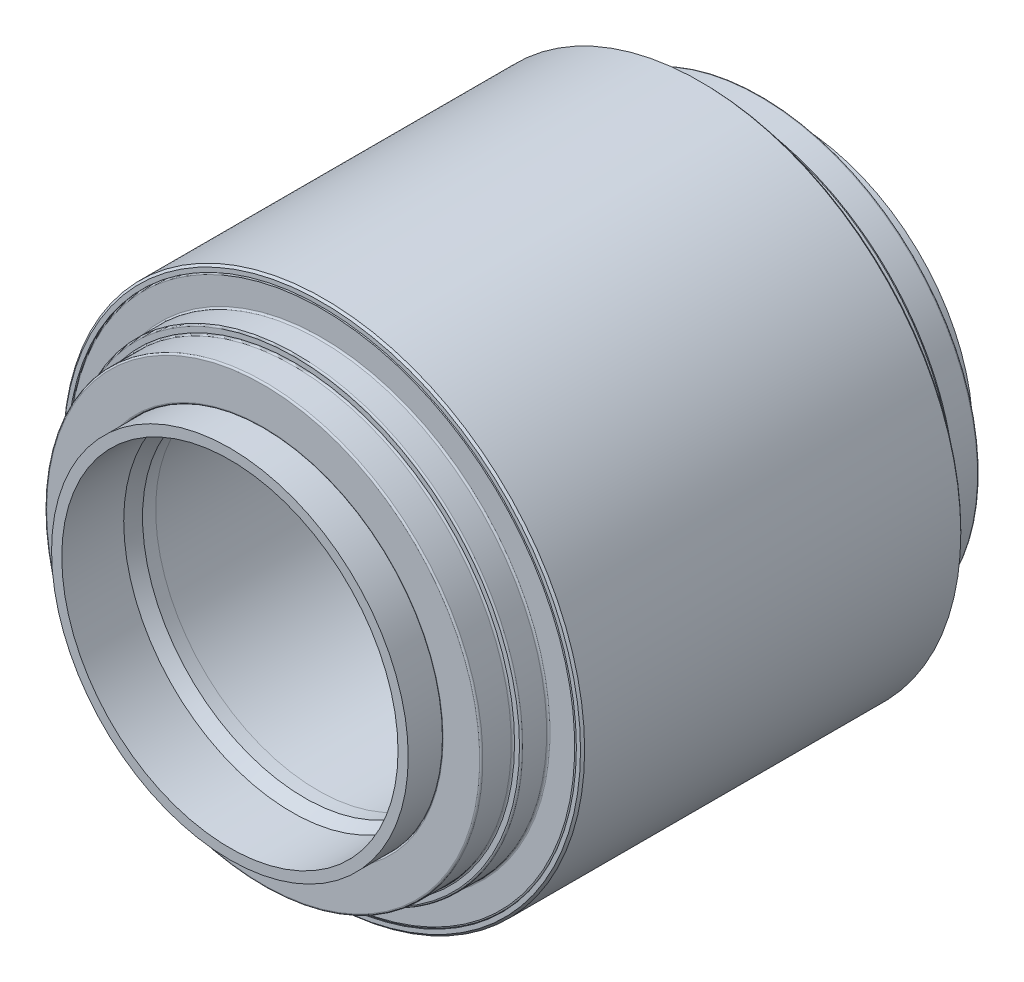
from build123d import *

# Parameters (mm, degrees)
SKETCH2_W          = 30
SKETCH2_H          = 5
SKETCH5_W          = 15.31
SKETCH5_H          = 17.764999952
SKETCH11_W         = 15.013
SKETCH11_H         = 17.764999952
FILLET1_R          = 0.8
FILLET2_R          = 0.8
CHAMFER1_SIZE      = 1
CIRPATTERN5_COUNT  = 26
CIRPATTERN7_COUNT  = 26
SKETCH15_R         = 3
CUT_EXTRUDE3_DEPTH = 225.788354196


with BuildPart() as part:
    # Sketch2 → Revolve1 (revolve)
    with BuildSketch(Plane(origin=(0, 0, 0), x_dir=(0, 0, -1), z_dir=(1, 0, 0)), mode=Mode.PRIVATE) as revolve1_sk:
        with Locations((0, 81.0749)):
            Rectangle(SKETCH2_W, SKETCH2_H)
    revolve(revolve1_sk.sketch.rotate(Axis((0, 0, 191.063546837), (0, 0, -1)), 90), axis=Axis((0, 0, 191.063546837), (0, 0, -1)))


with BuildPart() as body_2:
    # Sketch3 → Revolve2 (revolve)
    with BuildSketch(Plane(origin=(0, 0, 0), x_dir=(0, 0, -1), z_dir=(1, 0, 0)), mode=Mode.PRIVATE) as revolve2_sk:
        Polygon((-22.009341225, 88.613727462), (-71.184928734, 97.669414462), (-71.980821721, 93.5749), (-94.032, 93.5749), (-94.032, 78.5749), (-15, 78.5749), (-15, 86.5749), (-22.405649137, 86.5749), align=None)
    revolve(revolve2_sk.sketch.rotate(Axis((0, 0, 191.063546837), (0, 0, -1)), 90), axis=Axis((0, 0, 191.063546837), (0, 0, -1)))

    # Sketch7 → Revolve7 (revolve)
    with BuildSketch(Plane(origin=(0, 0, 0), x_dir=(0, 0, -1), z_dir=(-0.9927090359250009, 0.12053534748303266, 0)), mode=Mode.PRIVATE) as revolve7_sk:
        Polygon((-71.184928734, -96.95731027), (-22.009341225, -87.967647959), (-20.004670612, -98.205591502), (-69.086029785, -107.676482194), align=None)
    revolve7 = revolve(revolve7_sk.sketch.rotate(Axis((12.978822197, 106.891416831, 69.086029785), (-0.022837582945864243, -0.18808652749964044, -0.9818869094647906)), 353.201212474), axis=Axis((12.978822197, 106.891416831, 69.086029785), (-0.022837582945864243, -0.18808652749964044, -0.9818869094647906)))

    # CirPattern5: Revolve7 ×26 about axis
    cirpattern5_axis = Axis((0, 0, 191.063546837), (0, 0, -1))
    for i in range(1, CIRPATTERN5_COUNT):
        add(revolve7.rotate(cirpattern5_axis, i * 360 / CIRPATTERN5_COUNT))


with BuildPart() as body_3:
    # Sketch4 → Revolve3 (revolve)
    with BuildSketch(Plane(origin=(0, 0, 0), x_dir=(0, 0, -1), z_dir=(1, 0, 0)), mode=Mode.PRIVATE) as revolve3_sk:
        Polygon((-94.032, 78.5749), (-94.032, 85.485113365), (-104.032, 86.36), (-136.652, 86.36), (-136.652, 81.419999974), (-106.652, 81.419999974), (-100.382, 78.5749), align=None)
    revolve(revolve3_sk.sketch.rotate(Axis((0, 0, 191.063546837), (0, 0, -1)), 90), axis=Axis((0, 0, 191.063546837), (0, 0, -1)))


with BuildPart() as body_4:
    # Sketch5 → Revolve4 (revolve)
    with BuildSketch(Plane(origin=(0, 0, 0), x_dir=(0, 0, -1), z_dir=(1, 0, 0)), mode=Mode.PRIVATE) as revolve4_sk:
        with Locations((-111.39, 95.242499976)):
            Rectangle(SKETCH5_W, SKETCH5_H)
    revolve(revolve4_sk.sketch.rotate(Axis((0, 0, 191.063546837), (0, 0, -1)), 90), axis=Axis((0, 0, 191.063546837), (0, 0, -1)))


with BuildPart() as body_5:
    # Sketch6 → Revolve5 (revolve)
    with BuildSketch(Plane(origin=(0, 0, 0), x_dir=(0, 0, -1), z_dir=(1, 0, 0)), mode=Mode.PRIVATE) as revolve5_sk:
        Polygon((-78.915, 123.20625), (-78.915, 121.70625), (-90.575, 121.70625), (-90.575, 108.124999952), (-103.735, 108.124999952), (-103.735, 104.124999952), (-119.045, 104.124999952), (-119.045, 86.36), (-120.545, 86.36), (-120.545, 105.624999952), (-105.235, 105.624999952), (-105.235, 109.624999952), (-92.075, 109.624999952), (-92.075, 123.20625), align=None)
    revolve(revolve5_sk.sketch.rotate(Axis((0, 0, 191.063546837), (0, 0, -1)), 90), axis=Axis((0, 0, 191.063546837), (0, 0, -1)))

    # Fillet1
    fillet1_edges = [body_5.edges().sort_by_distance(p)[0] for p in [
        (-86.36, 0, 120.545),
        (-123.20625, 0, 92.075),
        (-109.624999952, 0, 92.075),
        (-109.624999952, 0, 105.235),
        (-105.624999952, 0, 105.235),
        (-105.624999952, 0, 120.545),
    ]]
    fillet(fillet1_edges, radius=FILLET1_R)


with BuildPart() as body_6:
    # Sketch9 → Revolve9 (revolve)
    with BuildSketch(Plane(origin=(0, 0, 0), x_dir=(0, 0, -1), z_dir=(1, 0, 0)), mode=Mode.PRIVATE) as revolve9_sk:
        Polygon((71.184928734, 97.669414462), (71.980821721, 93.5749), (94.032, 93.5749), (94.032, 78.5749), (15, 78.5749), (15, 86.5749), (22.405649137, 86.5749), (22.009341225, 88.613727462), align=None)
    revolve(revolve9_sk.sketch.rotate(Axis((0, 0, 191.063546837), (0, 0, -1)), 90), axis=Axis((0, 0, 191.063546837), (0, 0, -1)))

    # Sketch13 → Revolve13 (revolve)
    with BuildSketch(Plane(origin=(0, 0, 0), x_dir=(0, 0, -1), z_dir=(-0.9927090359250009, 0.12053534748303266, 0)), mode=Mode.PRIVATE) as revolve13_sk:
        Polygon((18.000787842, -108.444715529), (20.005652796, -98.205779473), (69.101665802, -107.601832375), (66.987918677, -118.396834602), align=None)
    revolve13 = revolve(revolve13_sk.sketch.rotate(Axis((11.837267754, 97.489764663, -20.005652796), (0.022657002110932568, 0.1865992938350363, -0.9821748132565867)), 173.199237638), axis=Axis((11.837267754, 97.489764663, -20.005652796), (0.022657002110932568, 0.1865992938350363, -0.9821748132565867)))

    # CirPattern7: Revolve13 ×26 about axis
    cirpattern7_axis = Axis((0, 0, 191.063546837), (0, 0, -1))
    for i in range(1, CIRPATTERN7_COUNT):
        add(revolve13.rotate(cirpattern7_axis, i * 360 / CIRPATTERN7_COUNT))


with BuildPart() as body_7:
    # Sketch10 → Revolve10 (revolve)
    with BuildSketch(Plane(origin=(0, 0, 0), x_dir=(0, 0, -1), z_dir=(1, 0, 0)), mode=Mode.PRIVATE) as revolve10_sk:
        Polygon((106.652, 81.419999974), (100.382, 78.5749), (94.032, 78.5749), (94.032, 85.485113365), (104.032, 86.36), (136.652, 86.36), (136.652, 81.419999974), align=None)
    revolve(revolve10_sk.sketch.rotate(Axis((0, 0, 191.063546837), (0, 0, -1)), 90), axis=Axis((0, 0, 191.063546837), (0, 0, -1)))

    # Sketch15 → Cut-Extrude3 (cut, through all)
    with BuildSketch(Plane(origin=(0, 0, 0), x_dir=(1, 0, 0), z_dir=(0, 1, 0))):
        with Locations((0, 136.652)):
            Circle(SKETCH15_R)
    extrude(amount=CUT_EXTRUDE3_DEPTH, mode=Mode.SUBTRACT)


with BuildPart() as body_8:
    # Sketch11 → Revolve11 (revolve)
    with BuildSketch(Plane(origin=(0, 0, 0), x_dir=(0, 0, -1), z_dir=(1, 0, 0)), mode=Mode.PRIVATE) as revolve11_sk:
        with Locations((111.5385, 95.242499976)):
            Rectangle(SKETCH11_W, SKETCH11_H)
    revolve(revolve11_sk.sketch.rotate(Axis((0, 0, 191.063546837), (0, 0, -1)), 90), axis=Axis((0, 0, 191.063546837), (0, 0, -1)))


with BuildPart() as body_9:
    # Sketch12 → Revolve12 (revolve)
    with BuildSketch(Plane(origin=(0, 0, 0), x_dir=(0, 0, -1), z_dir=(1, 0, 0)), mode=Mode.PRIVATE) as revolve12_sk:
        Polygon((120.545, 86.36), (119.045, 86.36), (119.045, 104.124999952), (103.735, 104.124999952), (103.735, 108.124999952), (90.575, 108.124999952), (90.575, 121.70625), (78.915, 121.70625), (78.915, 123.20625), (92.075, 123.20625), (92.075, 109.624999952), (105.235, 109.624999952), (105.235, 105.624999952), (120.545, 105.624999952), align=None)
    revolve(revolve12_sk.sketch.rotate(Axis((0, 0, 0), (0, 0, 1)), 90), axis=Axis((0, 0, 0), (0, 0, 1)))

    # Fillet2
    fillet2_edges = [body_9.edges().sort_by_distance(p)[0] for p in [
        (86.36, 0, -120.545),
        (105.624999952, 0, -120.545),
        (105.624999952, 0, -105.235),
        (109.624999952, 0, -105.235),
        (109.624999952, 0, -92.075),
        (123.20625, 0, -92.075),
    ]]
    fillet(fillet2_edges, radius=FILLET2_R)


with BuildPart() as body_10:
    # Sketch8 → Revolve8 (revolve)
    with BuildSketch(Plane(origin=(0, 0, 0), x_dir=(0, 0, -1), z_dir=(1, 0, 0)), mode=Mode.PRIVATE) as revolve8_sk:
        Polygon((-78.915, 123.20625), (-78.915, 121.70625), (-18, 109.23999996), (18, 109.23999996), (78.915, 121.70625), (78.915, 123.20625), (92.075, 123.20625), (92.075, 126.20625), (-92.075, 126.20625), (-92.075, 123.20625), align=None)
    revolve(revolve8_sk.sketch.rotate(Axis((0, 0, 191.063546837), (0, 0, -1)), 90), axis=Axis((0, 0, 191.063546837), (0, 0, -1)))

    # Chamfer1
    chamfer1_edges = [body_10.edges().sort_by_distance(p)[0] for p in [
        (-126.20625, 0, -92.075),
        (-126.20625, 0, 92.075),
    ]]
    chamfer(chamfer1_edges, length=CHAMFER1_SIZE)


solid = Compound([part.part, body_2.part, body_3.part, body_4.part, body_5.part, body_6.part, body_7.part, body_8.part, body_9.part, body_10.part])
